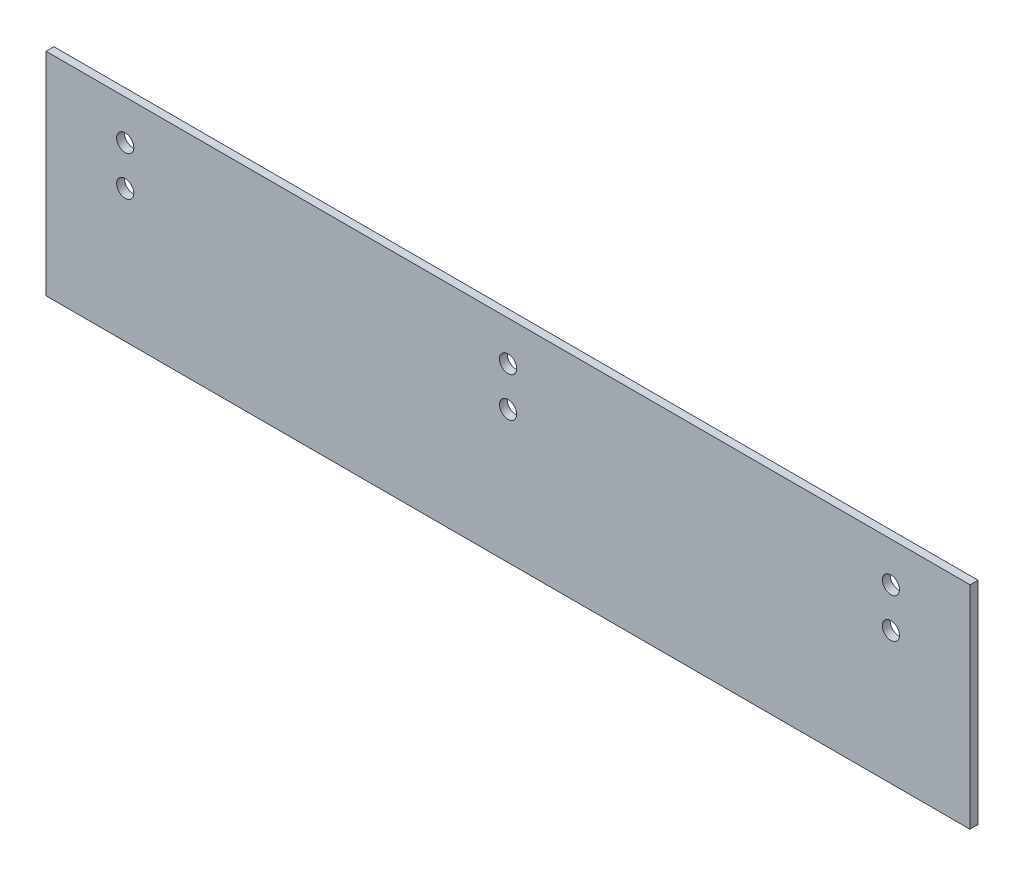
SolidWorks part; units mm, degrees
material "1023 碳钢板 (SS)"
ref_plane "前视基准面" through (0, 0, 0) normal (0, 0, 1) x (1, 0, 0)
ref_plane "上视基准面" through (0, 0, 0) normal (0, 1, 0) x (1, 0, 0)
ref_plane "右视基准面" through (0, 0, 0) normal (1, 0, 0) x (0, 0, -1)
sketch "草图1" plane through (0, 0, 0) normal (0, 0, 1) x (1, 0, 0)
  line L1 (-175, 42.5) -> (175, 42.5)
  line L2 (-175, 42.5) -> (-175, -42.5)
  line L3 (-175, -42.5) -> (175, -42.5)
  line L4 (175, 42.5) -> (175, -42.5)
  line L5 (-175, 42.5) -> (175, -42.5) construction
  line L6 (-175, -42.5) -> (175, 42.5) construction
  circle A0 centre (-145, 27.5) radius 3.25
  circle A1 centre (-145, 12.5) radius 3.25
  circle A2 centre (0, 27.5) radius 3.25
  circle A3 centre (0, 12.5) radius 3.25
  circle A4 centre (145, 27.5) radius 3.25
  circle A5 centre (145, 12.5) radius 3.25
  point P0 (0, 0)
  point P18 (0, 0)
  point P19 (0, 0)
  point P20 (0, 0)
  point P21 (0, 0)
  point P22 (0, 0)
  dimension "D8" = 6.5
  dimension "D1" = 350
  dimension "D2" = 85
  dimension "D3" = 30
  dimension "D4" = 145
  dimension "D5" = 30
  dimension "D6" = 15
  dimension "D7" = 15
extrude "凸台-拉伸1" add sketch "草图1" along normal blind 3
sketch "草图2" plane through (175, 0, 0) normal (1, 0, 0) x (0, 0, -1)
  line L0 (-3, 42.5) -> (0, 42.5) construction
  circle A0 centre (-1.5, -54.5) radius 16.85
  dimension "D2" = 33.7
  dimension "D1" = 97
extrude "切除-拉伸1" cut sketch "草图2" against normal blind 366
